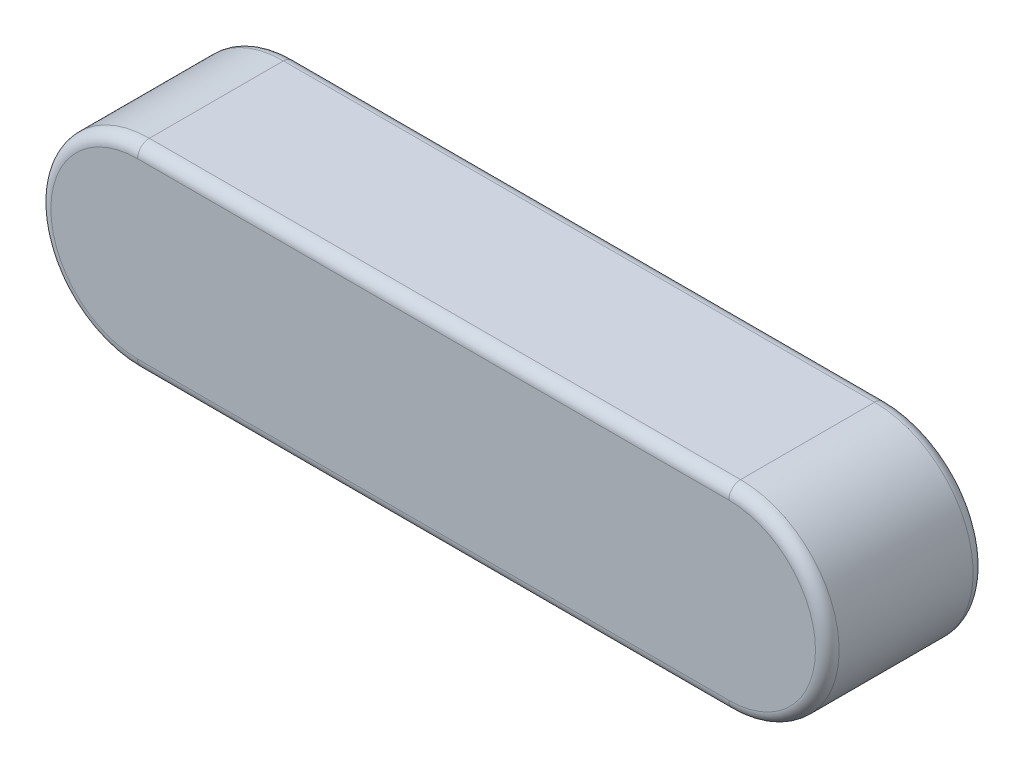
SolidWorks part; units mm, degrees
material "45"
ref_plane "基准面1" through (0, 0, 0) normal (0, 0, 1) x (1, 0, 0)
ref_plane "基准面2" through (0, 0, 0) normal (0, 1, 0) x (1, 0, 0)
ref_plane "基准面3" through (0, 0, 0) normal (1, 0, 0) x (0, 0, -1)
sketch "尺寸草图" plane through (0, 0, 0) normal (0, 0, 1) x (1, 0, 0)
  line L0 (-20, 0) -> (20, 0) construction
  point P3 (-8, 0)
  point P4 (-0.6, 0)
  point P5 (0, 0)
  point P8 (-10, 0)
  point P11 (0, 0)
sketch "草图1" plane through (0, 0, 0) normal (0, 0, 1) x (1, 0, 0)
  line L0 (-28.0599, 0) -> (30.562, 0) construction
  line L1 (-15, 5) -> (15, 5)
  line L2 (-15, -5) -> (15, -5)
  line L3 (0, 2.9108) -> (0, -2.1805) construction
  arc A0 (-15, 5) -> (-15, -5) centre (-15, 0) ccw
  arc A1 (15, 5) -> (15, -5) centre (15, 0) cw
extrude "基体-拉伸" add sketch "草图1" along normal blind 8
fillet "圆角1" radius 0.6 8 edges at (20, 0, 8) (0, 5, 8) (-20, 0, 8) (0, 5, 0) (20, 0, 0) (0, -5, 0) (-20, 0, 0) (0, -5, 8)
equation "\"D3@草图1\" = \"L@尺寸草图\""
equation "\"D1@草图1\" = \"b@尺寸草图\" / 2"
equation "\"D1@圆角1\" = \"r@尺寸草图\""
equation "\"D1@基体-拉伸\" = \"h@尺寸草图\""
